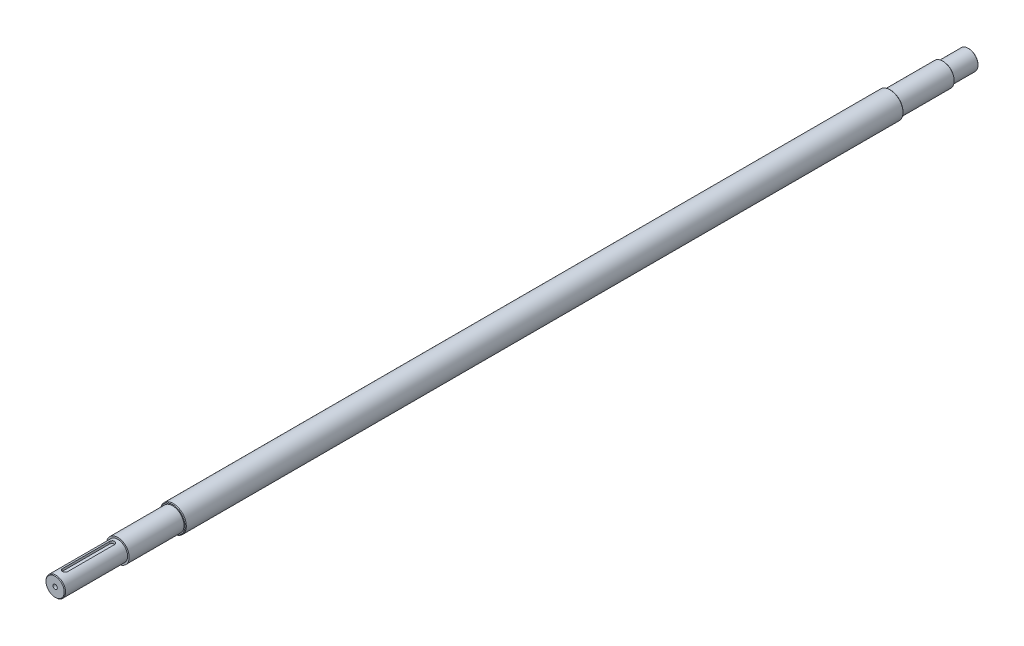
from build123d import *

# Parameters (mm, degrees)
SKETCH_2_R             = 15
EXTRUDE_1_DEPTH        = 96
SKETCH_3_R             = 17.5
EXTRUDE_2_DEPTH        = 84
SKETCH_4_R             = 20
EXTRUDE_3_DEPTH        = 1100
SKETCH_6_R             = 17.5
EXTRUDE_4_DEPTH        = 80
SKETCH_7_R             = 13
EXTRUDE_5_DEPTH        = 2
SKETCH_9_R             = 15
EXTRUDE_6_DEPTH        = 38
CHAMFER_1_SIZE         = 1
CHAMFER_2_SIZE         = 1
CHAMFER_3_SIZE         = 1
CHAMFER_4_SIZE         = 1
HOLE_WIZARD_M8_2_D     = 6.8
HOLE_WIZARD_M8_2_DEPTH = 28.75
HOLE_WIZARD_M8_2_TIP   = 2.042926105
CUT_EXTRUDE_1_DEPTH    = 1391.489482161


with BuildPart() as part:
    # 草图2 → 凸台-拉伸1 (new body)
    with BuildSketch(Plane.XY):
        Circle(SKETCH_2_R)
    extrude(amount=-EXTRUDE_1_DEPTH)

    # 草图3 → 凸台-拉伸2 (add)
    with BuildSketch(Plane(origin=(0, 0, -96), x_dir=(-1, 0, 0), z_dir=(0, 0, -1))):
        with Locations(Location((0, 0, 0), (0, 0, 180))):
            Circle(SKETCH_3_R)
    extrude(amount=EXTRUDE_2_DEPTH)

    # 草图4 → 凸台-拉伸3 (add)
    with BuildSketch(Plane(origin=(0, 0, -180), x_dir=(-1, 0, 0), z_dir=(0, 0, -1))):
        Circle(SKETCH_4_R)
    extrude(amount=EXTRUDE_3_DEPTH)

    # 草图6 → 凸台-拉伸4 (add)
    with BuildSketch(Plane(origin=(0, 0, -1280), x_dir=(-1, 0, 0), z_dir=(0, 0, -1))):
        with Locations(Location((0, 0, 0), (0, 0, 180))):
            Circle(SKETCH_6_R)
    extrude(amount=EXTRUDE_4_DEPTH)

    # 草图7 → 凸台-拉伸5 (add)
    with BuildSketch(Plane(origin=(0, 0, -1360), x_dir=(-1, 0, 0), z_dir=(0, 0, -1))):
        Circle(SKETCH_7_R)
    extrude(amount=EXTRUDE_5_DEPTH)

    # 草图9 → 凸台-拉伸6 (add)
    with BuildSketch(Plane(origin=(0, 0, -1362), x_dir=(-1, 0, 0), z_dir=(0, 0, -1))):
        with Locations(Location((0, 0, 0), (0, 0, 180))):
            Circle(SKETCH_9_R)
    extrude(amount=EXTRUDE_6_DEPTH)

    # 倒角1
    chamfer_1_edges = [part.edges().sort_by_distance(p)[0] for p in [
        (-15, 0, -1400),
    ]]
    chamfer(chamfer_1_edges, length=CHAMFER_1_SIZE)

    # 倒角2
    chamfer_2_edges = [part.edges().sort_by_distance(p)[0] for p in [
        (20, 0, -1280),
    ]]
    chamfer(chamfer_2_edges, length=CHAMFER_2_SIZE)

    # 倒角3
    chamfer_3_edges = [part.edges().sort_by_distance(p)[0] for p in [
        (20, 0, -180),
    ]]
    chamfer(chamfer_3_edges, length=CHAMFER_3_SIZE)

    # 倒角4
    chamfer_4_edges = [part.edges().sort_by_distance(p)[0] for p in [
        (-15, 0, 0),
    ]]
    chamfer(chamfer_4_edges, length=CHAMFER_4_SIZE)


with BuildPart() as part_1:
    # Move Body 1: moved
    add(part.part.moved(Location((0, 0, 10))))

    # M8 螺纹孔2
    with Locations(Plane.XY.offset(10)):
        with Locations((0, 0)):
            Hole(HOLE_WIZARD_M8_2_D / 2, depth=HOLE_WIZARD_M8_2_DEPTH)
            with Locations((0, 0, -(HOLE_WIZARD_M8_2_DEPTH + HOLE_WIZARD_M8_2_TIP / 2))):  # 118° drill point
                Cone(0, HOLE_WIZARD_M8_2_D / 2, HOLE_WIZARD_M8_2_TIP, mode=Mode.SUBTRACT)

    # 草图18 → 切除-拉伸1 (cut, through all)
    with BuildSketch(Plane(origin=(0, 11, 0), x_dir=(1, 0, 0), z_dir=(0, 1, 0))):
        with BuildLine():
            Line((4, 77), (4, 5))
            ThreePointArc((4, 5), (0, 1), (-4, 5))
            Line((-4, 5), (-4, 77))
            ThreePointArc((-4, 77), (0, 81), (4, 77))
        make_face()
    extrude(amount=CUT_EXTRUDE_1_DEPTH, mode=Mode.SUBTRACT)


solid = part_1.part
